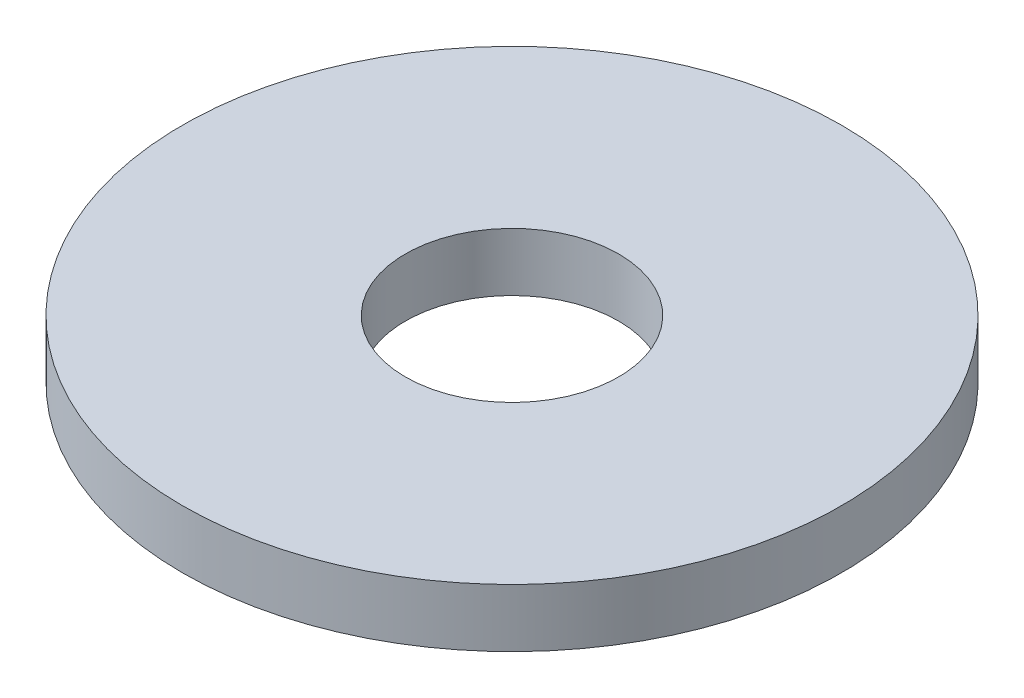
from build123d import *

# Parameters (mm, degrees)
SKETCH_1_W = 11.5
SKETCH_1_H = 3


with BuildPart() as part:
    # 草图1 → Revolve 468 (revolve)
    with BuildSketch(Plane.XY, mode=Mode.PRIVATE) as revolve_468_sk:
        with Locations((-11.25, 10.144507042)):
            Rectangle(SKETCH_1_W, SKETCH_1_H)
    revolve(revolve_468_sk.sketch.rotate(Axis((0, 0, 0), (0, 1, 0)), 270), axis=Axis((0, 0, 0), (0, 1, 0)))


solid = part.part
